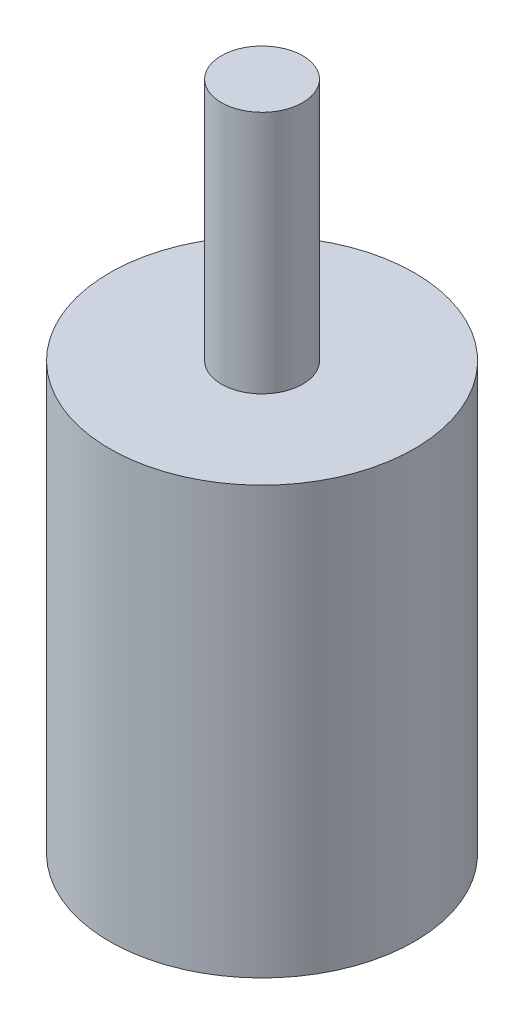
SolidWorks part; units mm, degrees
ref_plane "前视基准面" through (0, 0, 0) normal (0, 0, 1) x (1, 0, 0)
ref_plane "上视基准面" through (0, 0, 0) normal (0, 1, 0) x (1, 0, 0)
ref_plane "右视基准面" through (0, 0, 0) normal (1, 0, 0) x (0, 0, -1)
sketch "草图1" plane through (0, 0, 0) normal (0, 0, 1) x (1, 0, 0)
  line L0 (0, 0) -> (0, 6760.8664) construction
  line L1 (0, 11.2642) -> (2, 11.2642)
  line L2 (2, 11.2642) -> (2, -0.7358)
  line L3 (2, -0.7358) -> (7.5, -0.7358)
  line L4 (7.5, -0.7358) -> (7.5, -21.7358)
  line L5 (7.5, -21.7358) -> (0, -21.7358)
  line L6 (0, -21.7358) -> (0, 11.2642)
  dimension "D1" = 2
  dimension "D2" = 12
  dimension "D3" = 5.5
  dimension "D4" = 21
revolve "旋转1" add sketch "草图1" angle 360 about L0
